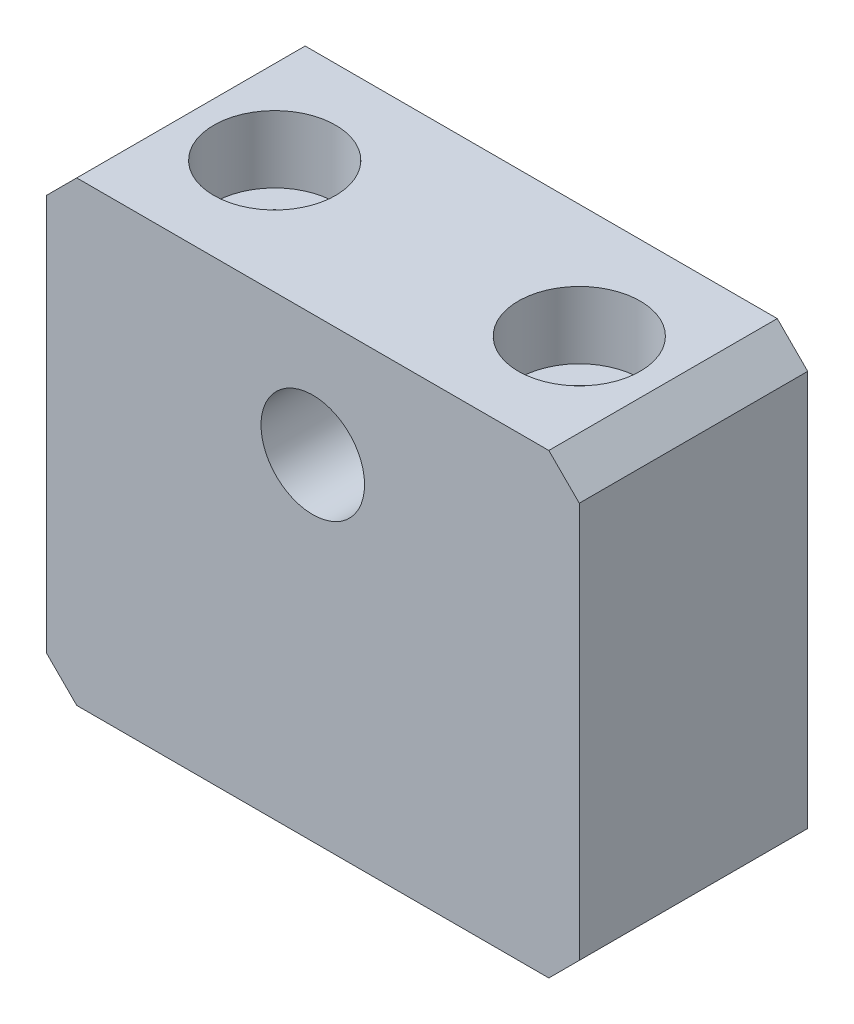
SolidWorks part; units mm, degrees
material "A6063"
ref_plane "Front Plane" through (0, 0, 0) normal (0, 0, 1) x (1, 0, 0)
ref_plane "Top Plane" through (0, 0, 0) normal (0, 1, 0) x (1, 0, 0)
ref_plane "Right Plane" through (0, 0, 0) normal (1, 0, 0) x (0, 0, -1)
sketch "Sketch1" plane through (0, 0, 0) normal (0, 0, 1) x (1, 0, 0)
  line L1 (-17.5, 15) -> (17.5, 15)
  line L2 (-17.5, 15) -> (-17.5, -15)
  line L3 (-17.5, -15) -> (17.5, -15)
  line L4 (17.5, 15) -> (17.5, -15)
  line L5 (-17.5, 15) -> (17.5, -15) construction
  line L6 (-17.5, -15) -> (17.5, 15) construction
  point P0 (0, 0)
  dimension "D1" = 35
  dimension "D2" = 30
extrude "Boss-Extrude1" add sketch "Sketch1" along normal blind 15
hole_wizard "CBORE for M4 Hex Socket Head Cap Screw1" positions "Sketch3" profile "Sketch2" counterbore size "M4" standard "Iso" end condition through all
sketch "Sketch3" plane through (0, 15, 0) normal (0, 1, 0) x (1, 0, 0)
  line L0 (-17.5, -7.5) -> (-17.7241, -7.5) construction
  line L1 (-17.5, -15) -> (-17.5, 0) construction
  line L3 (0, 0) -> (0, -15) construction
  line L4 (17.5, -15) -> (-17.5, -15) construction
  point P0 (-10, -7.5)
  point P17 (10, -7.5)
  dimension "D1" = 10
sketch "Sketch2" plane through (-10, 15, 7.5) normal (1, 0, 0) x (0, 0, 1)
  line L0 (0, 0) -> (0, 30)
  line L1 (0, 30) -> (2.25, 30)
  line L3 (2.25, 30) -> (2.25, 4.4)
  line L4 (2.25, 4.4) -> (4, 4.4)
  line L5 (4, 4.4) -> (4, 0)
  line L7 (4, 0) -> (0, 0)
  line L11 (0, -6.35) -> (0, 107.95) construction
  dimension "通孔孔直径" = 4.5
  dimension "通孔孔深度" = 30
  dimension "柱形沉头孔直径" = 8
  dimension "柱形沉头孔深度" = 4.4
hole_wizard "M8 Tapped Hole1" positions "Sketch5" profile "Sketch4" tap size "M8" standard "Gb"
sketch "Sketch5" plane through (0, 0, 15) normal (0, 0, 1) x (1, 0, 0)
  line L0 (0, 15) -> (0, -15) construction
  line L1 (17.5, 15) -> (-17.5, 15) construction
  line L2 (-17.5, -15) -> (17.5, -15) construction
  point P0 (0, 7)
  dimension "D1" = 22
sketch "Sketch4" plane through (0, 7, 15) normal (1, 0, 0) x (0, -1, 0)
  line L0 (0, 0) -> (0, 24.2929)
  line L1 (0, 24.2929) -> (3.4, 22.25)
  line L2 (3.4, 22.25) -> (3.4, 0)
  line L5 (3.4, 0) -> (0, 0)
  line L10 (0, 24.2929) -> (-3.4, 22.25) construction
  line L11 (0, -6.35) -> (0, 107.95) construction
  dimension "螺纹孔钻头直径" = 6.8
  dimension "螺纹孔钻头深度" = 22.25
  dimension "导头角度" = 118
cosmetic thread "Cosmetic thread 1" parameters "D1"=15, "D2"=8
chamfer "Chamfer1" distance 2 angle 45 4 edges at (-17.5, -15, 7.5) (17.5, -15, 7.5) (17.5, 15, 7.5) (-17.5, 15, 7.5)
